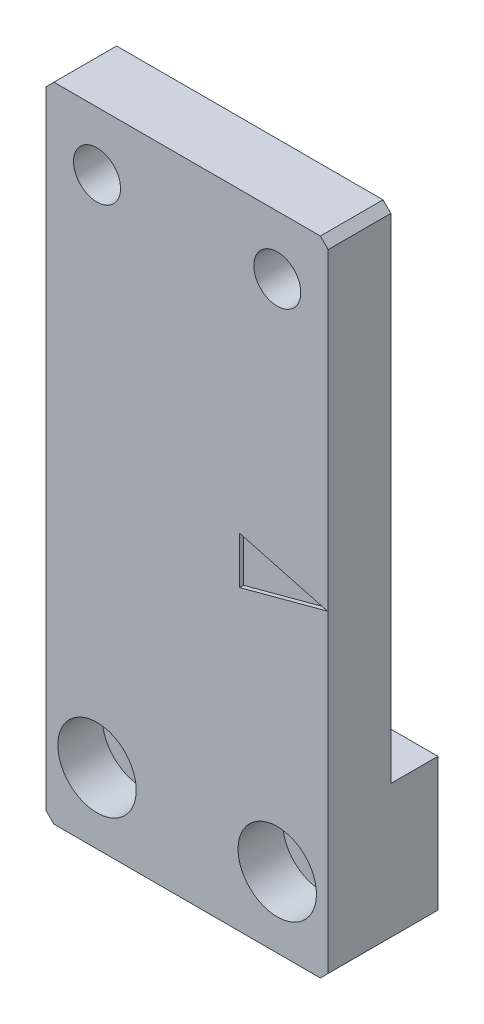
from build123d import *

# Parameters (mm, degrees)
BOSS_EXTRUDE1_DEPTH                                  = 18
HOLE_SIZE_PER_SOCKET_HEAD_CAP_SCREW_TYPE_D           = 5.5
HOLE_SIZE_PER_SOCKET_HEAD_CAP_SCREW_TYPE_CBORE_D     = 10
HOLE_SIZE_PER_SOCKET_HEAD_CAP_SCREW_TYPE_CBORE_DEPTH = 5.7
SKETCH5_R                                            = 3
CUT_EXTRUDE1_DEPTH                                   = 86.111691324
CHAMFER1_SIZE                                        = 1
CUT_EXTRUDE3_DEPTH                                   = 0.5


with BuildPart() as part:
    # Sketch1 → Boss-Extrude1 (new, symmetric)
    with BuildSketch(Plane(origin=(0, 0, 0), x_dir=(0, 0, -1), z_dir=(1, 0, 0))):
        Polygon((14, 0), (0, 0), (0, 82), (8, 82), (8, 18), (14, 18), align=None)
    extrude(amount=BOSS_EXTRUDE1_DEPTH, both=True)

    # Hole size per socket head cap screw type1 (through all)
    with Locations(Plane.XY):
        with Locations((11.5, 9), (-11.5, 9)):
            CounterBoreHole(HOLE_SIZE_PER_SOCKET_HEAD_CAP_SCREW_TYPE_D / 2, HOLE_SIZE_PER_SOCKET_HEAD_CAP_SCREW_TYPE_CBORE_D / 2, HOLE_SIZE_PER_SOCKET_HEAD_CAP_SCREW_TYPE_CBORE_DEPTH)

    # Sketch5 → Cut-Extrude1 (cut, through all)
    with BuildSketch(Plane.XY):
        with Locations((-11.5, 74.5)):
            Circle(SKETCH5_R)
        with Locations(Location((11.5, 74.5, 0), (0, 0, 270))):
            Circle(SKETCH5_R)
    extrude(amount=-CUT_EXTRUDE1_DEPTH, mode=Mode.SUBTRACT)

    # Chamfer1
    chamfer1_edges = [part.edges().sort_by_distance(p)[0] for p in [
        (18, 82, -4),
        (18, 0, -7),
        (-18, 0, -7),
        (-18, 82, -4),
    ]]
    chamfer(chamfer1_edges, length=CHAMFER1_SIZE)

    # Sketch6 → Cut-Extrude3 (cut)
    with BuildSketch(Plane.XY):
        Polygon((6.7, 44), (17.896152423, 41), (6.7, 38), align=None)
    extrude(amount=-CUT_EXTRUDE3_DEPTH, mode=Mode.SUBTRACT)


solid = part.part
